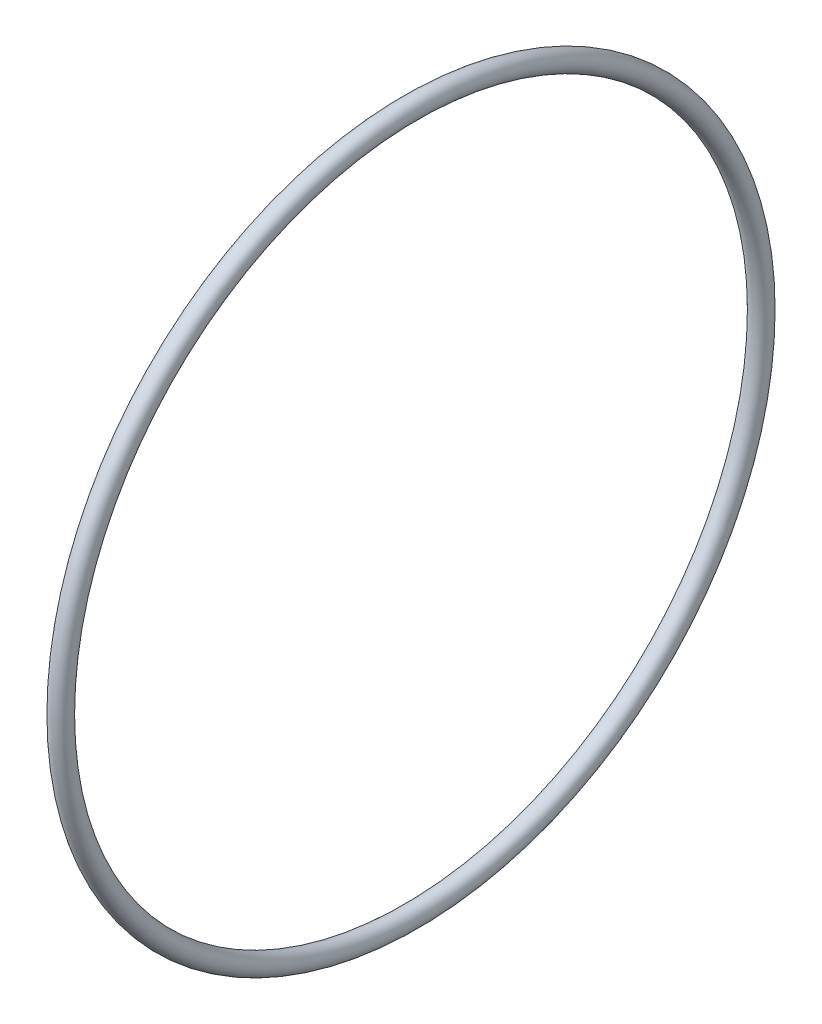
from build123d import *

# Parameters (mm, degrees)
SKETCH1_R = 1.325


with BuildPart() as part:
    # Sketch1 → Revolve1 (revolve)
    with BuildSketch(Plane.XY, mode=Mode.PRIVATE) as revolve1_sk:
        with Locations((5, 47.35)):
            Circle(SKETCH1_R)
    revolve(revolve1_sk.sketch.rotate(Axis((0, 0, 0), (1, 0, 0)), 90), axis=Axis((0, 0, 0), (1, 0, 0)))


solid = part.part
